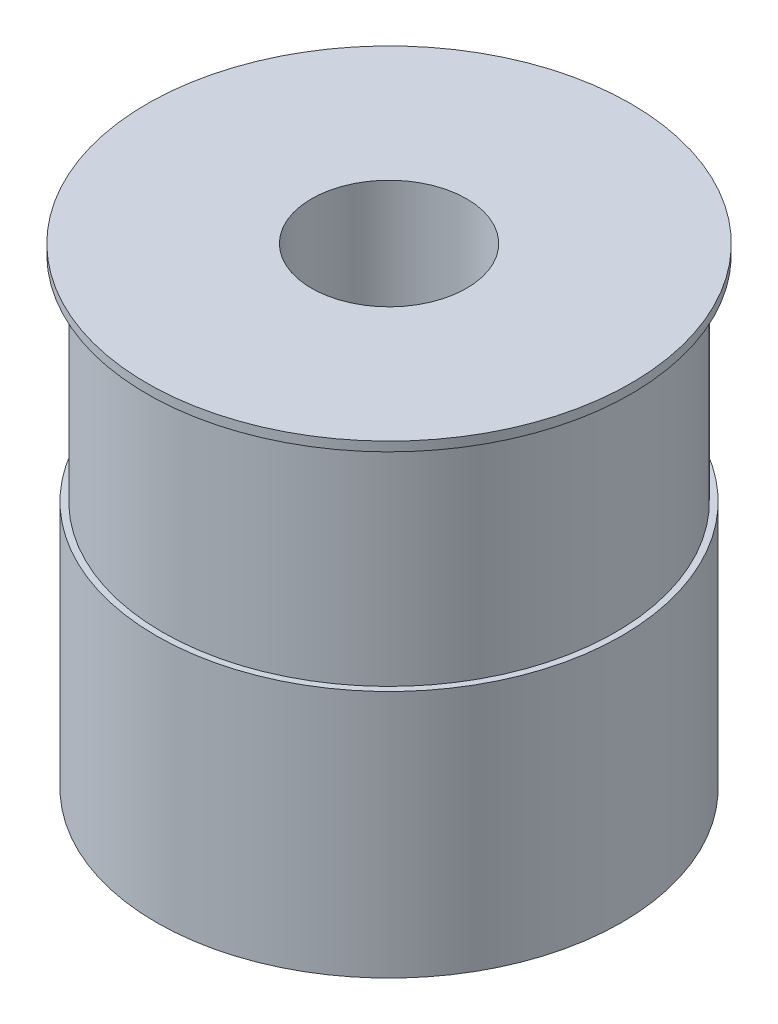
SolidWorks part; units mm, degrees
ref_plane "前视基准面" through (0, 0, 0) normal (0, 0, 1) x (1, 0, 0)
ref_plane "上视基准面" through (0, 0, 0) normal (0, 1, 0) x (1, 0, 0)
ref_plane "右视基准面" through (0, 0, 0) normal (1, 0, 0) x (0, 0, -1)
sketch "草图1" plane through (0, 0, 0) normal (0, 0, 1) x (1, 0, 0)
  line L0 (0, 0) -> (0, 73.125) construction
  line L1 (0, 0) -> (-37.5, 0) construction
  line L2 (-37.5, 0) -> (-37.5, 40)
  line L3 (-37.5, 40) -> (-36.5, 40)
  line L4 (-36.5, 40) -> (-36.5, 74.5)
  line L5 (-36.5, 74.5) -> (-39, 74.5)
  line L6 (-39, 74.5) -> (-39, 76)
  line L7 (-39, 76) -> (-17.5, 76)
  line L8 (-37.5, 0) -> (-32.5, 0)
  line L9 (-32.5, 0) -> (-32.5, 33)
  line L10 (-32.5, 33) -> (-30, 33)
  line L11 (-30, 33) -> (-30, 36)
  line L12 (-30, 36) -> (-17.5, 36)
  line L13 (-17.5, 36) -> (-17.5, 76) construction
  line L14 (-17.5, 36) -> (-17.5, 51)
  line L15 (-17.5, 51) -> (-12.5, 51)
  line L16 (-12.5, 51) -> (-12.5, 76)
  line L17 (-12.5, 76) -> (-17.5, 76)
  dimension "D2" = 5
  dimension "D3" = 76
  dimension "D4" = 60
  dimension "D5" = 33
  dimension "D6" = 12.5
  dimension "D7" = 4
  dimension "D8" = 1
  dimension "D9" = 40
  dimension "D10" = 1.5
  dimension "D11" = 1.5
  dimension "D12" = 32.5
  dimension "D13" = 15
  dimension "D14" = 5
revolve "旋转1" add sketch "草图1" angle 360 about L0
equation "\"图号代码1\"= \"图号代码\""
equation "\"名称代码2\"= \"名称代码\""
